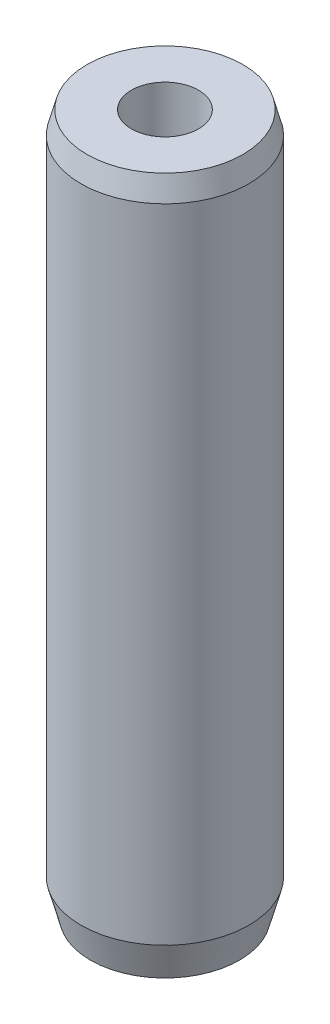
SolidWorks part; units mm, degrees
material "35"
ref_plane "Front Plane" through (0, 0, 0) normal (0, 0, 1) x (1, 0, 0)
ref_plane "Top Plane" through (0, 0, 0) normal (0, 1, 0) x (1, 0, 0)
ref_plane "Right Plane" through (0, 0, 0) normal (1, 0, 0) x (0, 0, -1)
sketch "Sketch1" plane through (0, 0, 0) normal (0, 1, 0) x (1, 0, 0)
  circle A0 centre (0, 0) radius 6
  dimension "D1" = 12
extrude "Boss-Extrude1" add sketch "Sketch1" along normal mid plane 50
hole_wizard "M6 Tapped Hole1" positions "Sketch3" profile "Sketch2" tap size "M6" standard "GB"
sketch "Sketch3" plane through (0, 25, 0) normal (0, 1, 0) x (1, 0, 0)
  point P0 (0, 0)
sketch "Sketch2" plane through (0, 25, 0) normal (1, 0, 0) x (0, 0, 1)
  line L0 (0, 0) -> (0, 21.3856)
  line L1 (0, 21.3856) -> (2.4, 20)
  line L2 (2.4, 20) -> (2.4, 0)
  line L5 (2.4, 0) -> (0, 0)
  line L10 (0, 21.3856) -> (-2.4, 20) construction
  line L11 (0, -6.35) -> (0, 107.95) construction
  dimension "螺纹孔钻头直径" = 4.8
  dimension "螺纹孔钻头深度" = 20
  dimension "导头角度" = 120
cosmetic thread "Cosmetic Thread1" parameters "D1"=12, "D2"=6
chamfer "Chamfer1" distance 1.6 angle 15 1 edges at (0, 25, 6)
chamfer "Chamfer2" distance 2.5 angle 15 1 edges at (0, -25, 6)
